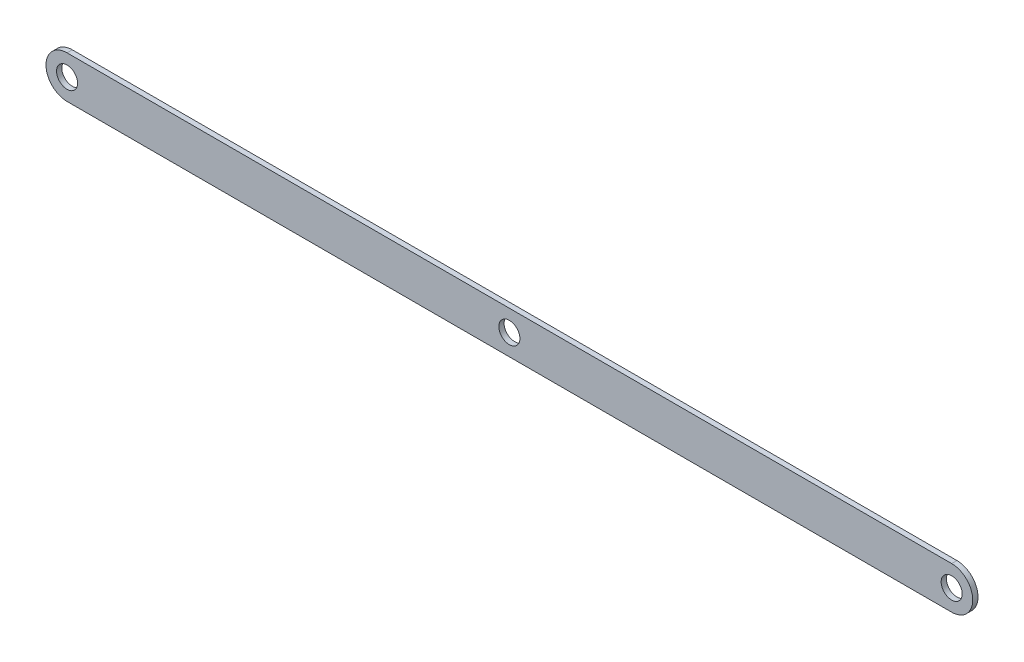
from build123d import *

# Parameters (mm, degrees)
SKETCH1_R           = 5
BOSS_EXTRUDE1_DEPTH = 2.5


with BuildPart() as part:
    # Sketch1 → Boss-Extrude1 (new body)
    with BuildSketch(Plane.XY):
        with BuildLine():
            Line((-210, 10), (210, 10))
            ThreePointArc((210, 10), (220, 0), (210, -10))
            Line((210, -10), (-210, -10))
            ThreePointArc((-210, -10), (-220, 0), (-210, 10))
        make_face()
        with Locations((-210, 0)):
            Circle(SKETCH1_R, mode=Mode.SUBTRACT)
        with Locations((210, 0)):
            Circle(SKETCH1_R, mode=Mode.SUBTRACT)
        Circle(SKETCH1_R, mode=Mode.SUBTRACT)
    extrude(amount=BOSS_EXTRUDE1_DEPTH)


solid = part.part
